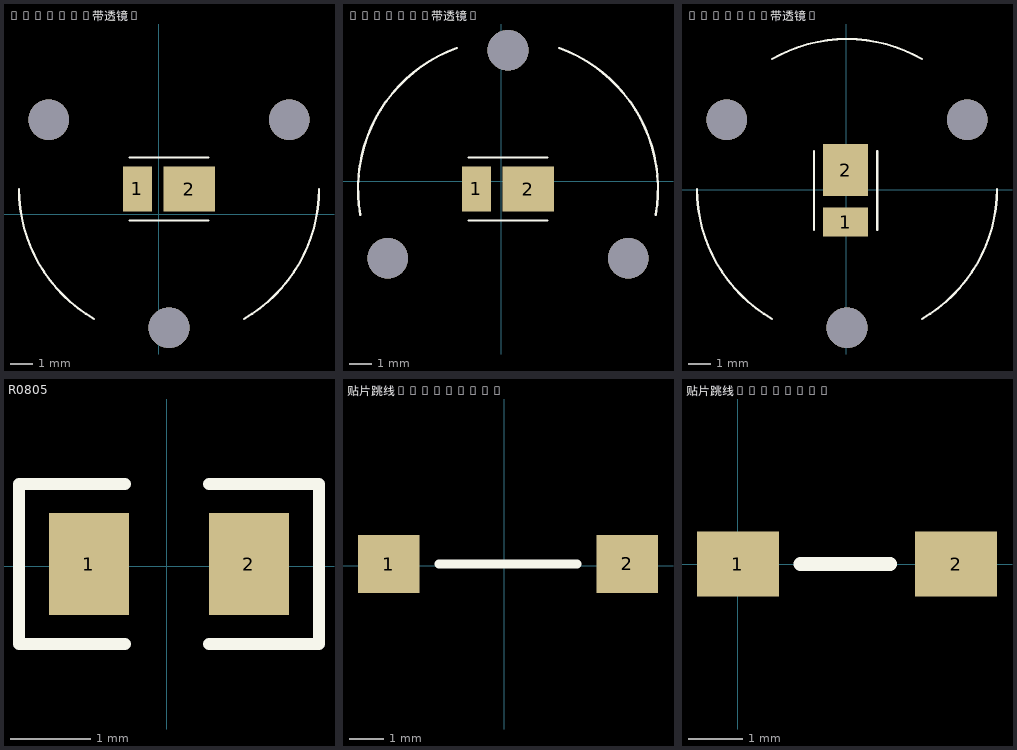
[diagram p0: the footprints below, top view; thin cyan lines are the x and y axes]
# Altium footprint library MISC59163-2.PcbLib: 6 footprints
Each footprint in its own frame and in the unit in brackets; x right, y up, seen from the top. Pads: shape width x height; smd on the part's side, far side on the other; paste and mask are expansions set on the pad; w line width, h text height; cw(c..) or ccw(c..) is an arc to the next point about the centre after c.

## 2835LED带透镜1 [mm]
pads (2):
  rect 1.3x2 smd: 1(-0.95,1.125)
  rect 2.3x2 smd: 2(1.35,1.125)
via 5.776,4.2 diameter 1.8 hole 1.8
via 0.45,-5.025 diameter 1.8 hole 1.8
via -4.876,4.2 diameter 1.8 hole 1.8
Top Overlay:
  lines w0.1: -6.2,1.125 ccw(c0.45,1.125) -2.875,-4.634 ; -1.3,-0.275 2.2,-0.275 ; -1.3,2.525 2.2,2.525 ; 3.775,-4.634 ccw(c0.45,1.125) 7.1,1.125

## 2835LED带透镜2 [mm]
pads (2):
  rect 1.3x2 smd: 1(-1.102,-0.35)
  rect 2.3x2 smd: 2(1.198,-0.35)
via 0.298,5.8 diameter 1.8 hole 1.8
via 5.624,-3.425 diameter 1.8 hole 1.8
via -5.028,-3.425 diameter 1.8 hole 1.8
Top Overlay:
  lines w0.1: -6.251,-1.505 cw(c0.298,-0.35) -1.976,5.899 ; -1.452,-1.75 2.048,-1.75 ; -1.452,1.05 2.048,1.05 ; 2.572,5.899 cw(c0.298,-0.35) 6.847,-1.505

## 2835LED带透镜3 [mm]
pads (2):
  rect 2x1.3 smd: 1(-0.029,-1.433)
  rect 2x2.3 smd: 2(-0.029,0.867)
via 5.355,3.108 diameter 1.8 hole 1.8
via 0.029,-6.117 diameter 1.8 hole 1.8
via -5.297,3.108 diameter 1.8 hole 1.8
Top Overlay:
  lines w0.1: -6.621,0.033 ccw(c0.029,0.033) -3.296,-5.726 ; -3.296,5.792 cw(c0.029,0.033) 3.354,5.792 ; -1.429,-1.783 -1.429,1.717 ; 1.371,-1.783 1.371,1.717 ; 3.354,-5.726 ccw(c0.029,0.033) 6.679,0.033

## R0805 [mm]
pads (2):
  rect 1x1.27 smd: 1(-0.975,0.025) 2(1.025,0.025)
Top Overlay:
  lines w0: -0.525,0.975 -0.512,0.963 ; -0.525,-0.925 -0.525,-0.925
  lines w0.15: -0.525,-0.975 -1.85,-0.975 -1.85,1.025 -0.525,1.025 ; 0.525,-0.975 1.9,-0.975 1.9,1.025 0.525,1.025

## 贴片跳线QM8.2-D01 [mm]
pads (2):
  rect 1.8x1.7 smd: 1(-3.389,0.054) 2(3.611,0.054)
Top Overlay:
  lines w0.254: -1.921,0.054 2.143,0.054

## 贴片跳线QM52-D01 [mm]
pads (2):
  rect 1.5x1.2 smd: 1(0,0) 2(4,0)
Top Overlay:
  lines w0.254: 1.143,0 2.794,0